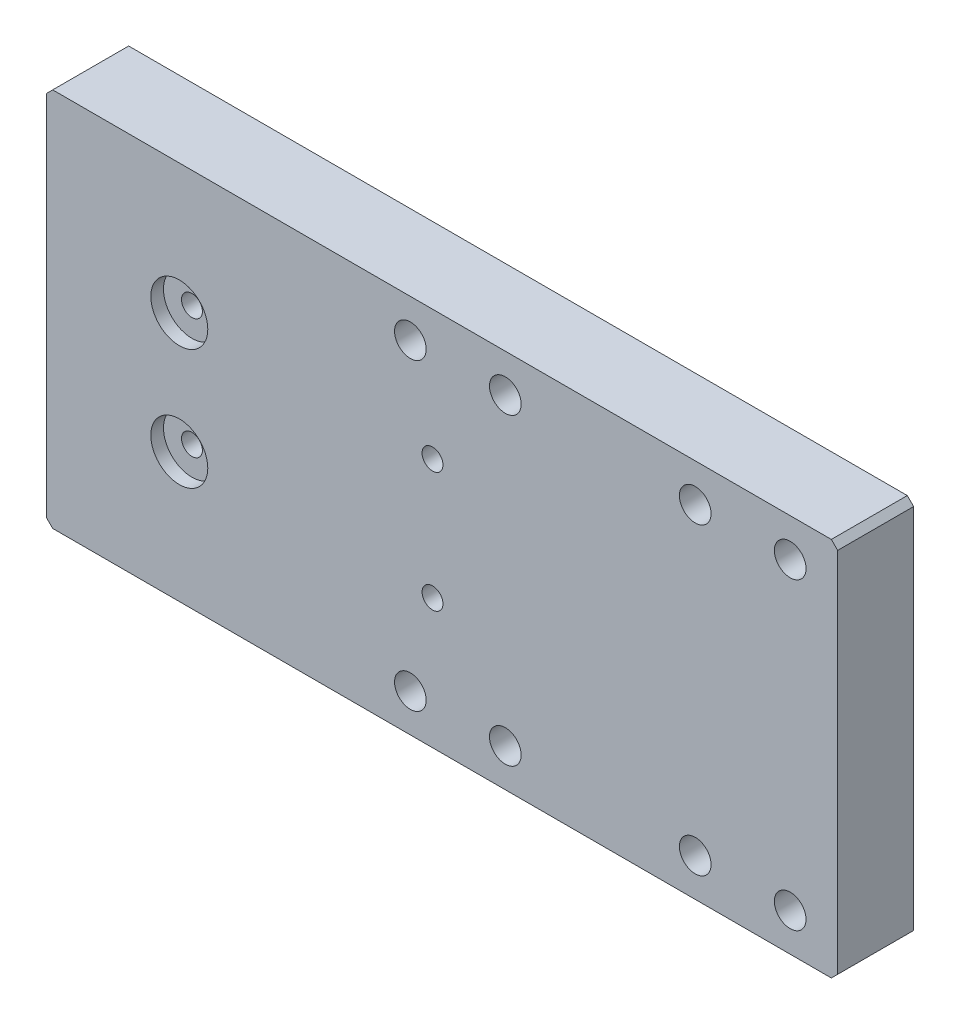
from build123d import *

# Parameters (mm, degrees)
SKETCH1_W                 = 125
SKETCH1_H                 = 60
BOSS_EXTRUDE1_DEPTH       = 6
M6_TAPPED_HOLE1_D         = 5
M4_TAPPED_HOLE1_D         = 3.3
SKETCH8_R                 = 4.5
CUT_EXTRUDE1_DEPTH        = 2
BLIND_PIN_HOLE1_SIZE_MM_D = 5
CHAMFER1_SIZE             = 1


with BuildPart() as part:
    # Sketch1 → Boss-Extrude1 (new, symmetric)
    with BuildSketch(Plane.XY):
        Rectangle(SKETCH1_W, SKETCH1_H)
    extrude(amount=BOSS_EXTRUDE1_DEPTH, both=True)

    # M6 Tapped Hole1 (through all)
    with Locations(Plane(origin=(0, 0, -6), x_dir=(-1, 0, 0), z_dir=(0, 0, -1))):
        with Locations((5, 24), (5, -24), (-55, -24), (-55, 24)):
            Hole(M6_TAPPED_HOLE1_D / 2)

    # M4 Tapped Hole1 (through all)
    with Locations(Plane.XY.offset(6)):
        with Locations((-1.5, 9.5), (-1.5, -9.5), (-41.5, -9.5), (-41.5, 9.5)):
            Hole(M4_TAPPED_HOLE1_D / 2)

    # Sketch8 → Cut-Extrude1 (cut)
    with BuildSketch(Plane.XY.offset(6)):
        with Locations((-41.5, 9.5)):
            Circle(SKETCH8_R)
        with Locations((-41.5, -9.5)):
            Circle(SKETCH8_R)
    extrude(amount=-CUT_EXTRUDE1_DEPTH, mode=Mode.SUBTRACT)

    # Blind Pin Hole1 (size mm) (through all)
    with Locations(Plane.XY.offset(6)):
        with Locations((10, 24), (40, 24), (10, -24), (40, -24)):
            Hole(BLIND_PIN_HOLE1_SIZE_MM_D / 2)

    # Chamfer1
    chamfer1_edges = [part.edges().sort_by_distance(p)[0] for p in [
        (62.5, -30, 0),
        (-62.5, -30, 0),
        (-62.5, 30, 0),
        (62.5, 30, 0),
    ]]
    chamfer(chamfer1_edges, length=CHAMFER1_SIZE)


solid = part.part
